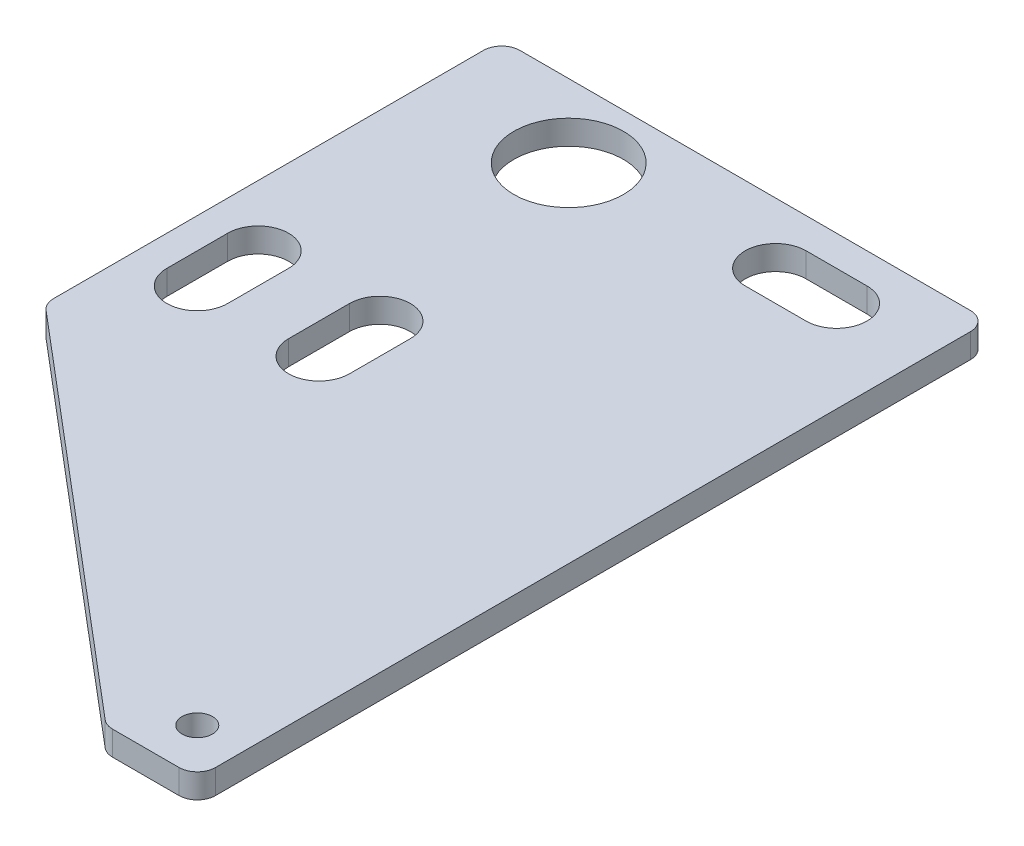
from build123d import *

# Parameters (mm, degrees)
SKETCH1_R           = 9
SKETCH1_R_2         = 2.5
BOSS_EXTRUDE1_DEPTH = 4
FILLET1_R           = 3


with BuildPart() as part:
    # Sketch1 → Boss-Extrude1 (new body)
    with BuildSketch(Plane(origin=(0, 0, 0), x_dir=(1, 0, 0), z_dir=(0, 1, 0))):
        Polygon((0, 0), (-80, 0), (-80, -75), (-15, -130), (0, -130), align=None)
        with Locations(Location((-57, -12, 0), (0, 0, 270))):
            Circle(SKETCH1_R, mode=Mode.SUBTRACT)
        with Locations(Location((-7.5, -122.5, 0), (0, 0, 270))):
            Circle(SKETCH1_R_2, mode=Mode.SUBTRACT)
        with BuildLine():
            Line((-25, -5), (-15, -5))
            ThreePointArc((-15, -5), (-10, -10), (-15, -15))
            Line((-15, -15), (-25, -15))
            ThreePointArc((-25, -15), (-30, -10), (-25, -5))
        make_face(mode=Mode.SUBTRACT)
        with BuildLine():
            Line((-65, -50), (-65, -60))
            ThreePointArc((-65, -60), (-70, -65), (-75, -60))
            Line((-75, -60), (-75, -50))
            ThreePointArc((-75, -50), (-70, -45), (-65, -50))
        make_face(mode=Mode.SUBTRACT)
        with BuildLine():
            Line((-45, -50), (-45, -60))
            ThreePointArc((-45, -60), (-50, -65), (-55, -60))
            Line((-55, -60), (-55, -50))
            ThreePointArc((-55, -50), (-50, -45), (-45, -50))
        make_face(mode=Mode.SUBTRACT)
    extrude(amount=BOSS_EXTRUDE1_DEPTH)

    # Fillet1
    fillet1_edges = [part.edges().sort_by_distance(p)[0] for p in [
        (0, 2, 130),
        (-15, 2, 130),
        (-80, 2, 75),
        (-80, 2, 0),
        (0, 2, 0),
    ]]
    fillet(fillet1_edges, radius=FILLET1_R)


solid = part.part
